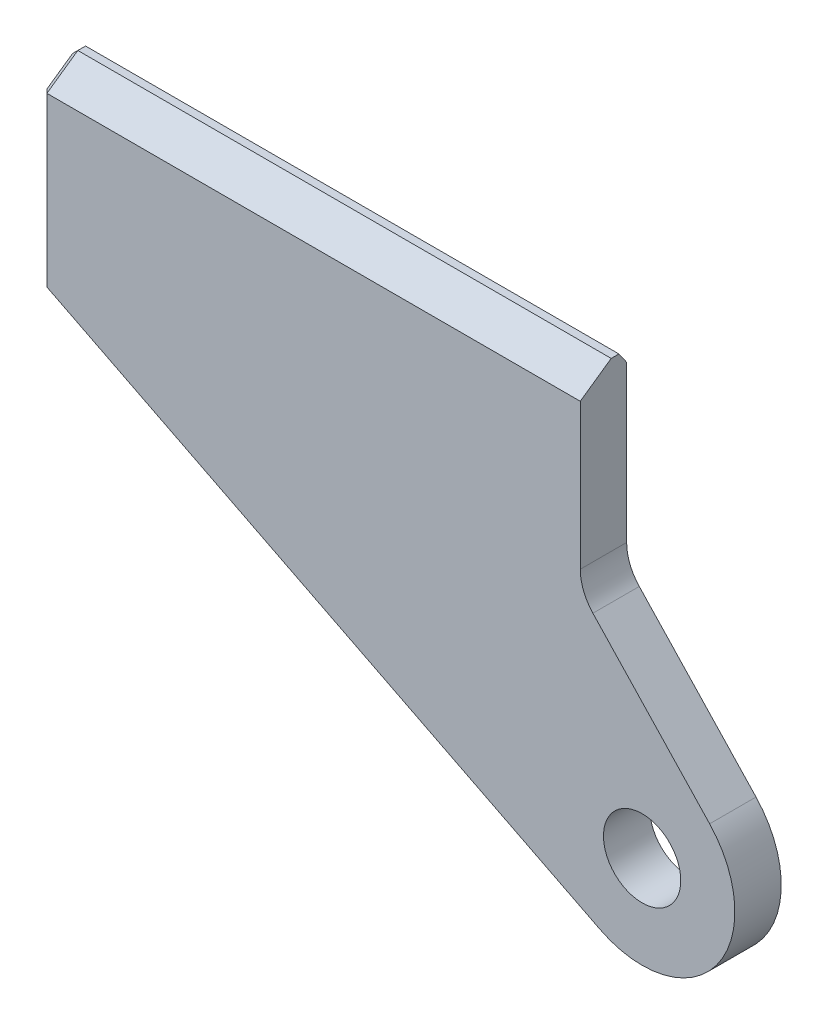
SolidWorks part; units mm, degrees
material "Q345"
ref_plane "前视基准面" through (0, 0, 0) normal (0, 0, 1) x (1, 0, 0)
ref_plane "上视基准面" through (0, 0, 0) normal (0, 1, 0) x (1, 0, 0)
ref_plane "右视基准面" through (0, 0, 0) normal (1, 0, 0) x (0, 0, -1)
sketch "草图1" plane through (0, 0, 0) normal (0, 0, 1) x (1, 0, 0)
  line L0 (-40, 250) -> (-390, 250)
  line L1 (-390, 250) -> (-390, 130)
  line L2 (60, 0) -> (60, 250) construction
  line L3 (-390, 130) -> (-27.0782, -53.5422)
  line L5 (-40, 250) -> (60, 250) construction
  line L6 (-40, 250) -> (-40, 130)
  line L7 (-40, 130) -> (43.6817, 41.1328)
  line L8 (-390, 130) -> (-40, 130) construction
  circle A0 centre (0, 0) radius 25
  arc A1 (-27.0782, -53.5422) -> (43.6817, 41.1328) centre (0, 0) ccw
  circle A2 centre (0, 0) radius 60 construction
  dimension "D1" = 50
  dimension "D2" = 120
  dimension "D3" = 450
  dimension "D4" = 250
  dimension "D5" = 120
  dimension "D6" = 100
extrude "凸台-拉伸1" add sketch "草图1" along normal blind 30
ref_plane "基准面1" through (60, 0, 0) normal (1, 0, 0) x (0, 0, -1)
sketch "草图2" plane through (60, 0, 0) normal (1, 0, 0) x (0, 0, -1)
  line L0 (-10, 250) -> (-30, 235.9958)
  line L3 (0, 130) -> (0, 250) construction
  line L7 (-10, 250) -> (-30, 250)
  line L8 (-30, 250) -> (-30, 235.9958)
  dimension "D1" = 10
  dimension "D2" = 55
extrude "切除-拉伸2" cut sketch "草图2" against normal through all
sketch "草图3" plane through (60, 0, 0) normal (1, 0, 0) x (0, 0, -1)
  line L0 (-5, 250) -> (0, 242.8593)
  line L6 (-5, 250) -> (0, 250)
  line L7 (0, 250) -> (0, 242.8593)
  line L10 (-10, 250) -> (0, 250) construction
  line L11 (-10, 250) -> (-30, 235.9958) construction
extrude "切除-拉伸3" cut sketch "草图3" against normal through all
chamfer "倒角1" distance 5 angle 45 5 edges at (-390, 182.9979, 30) (-390, 242.9979, 20) (-390, 250, 7.5) (-390, 246.4296, 2.5) (-390, 186.4296, 0)
sketch "草图5" plane through (0, 0, 0) normal (0, 0, -1) x (-1, 0, 0)
  circle A0 centre (0, 0) radius 49
  circle A1 centre (0, 49) radius 4
  circle A2 centre (42.4352, -24.5) radius 4
  circle A3 centre (-42.4352, -24.5) radius 4
  point P11 (0, 0)
  dimension "D1" = 98
  dimension "D2" = 8
  dimension "D3" = 3
fillet "圆角2" radius 30 1 edges at (-40, 130, 15)
